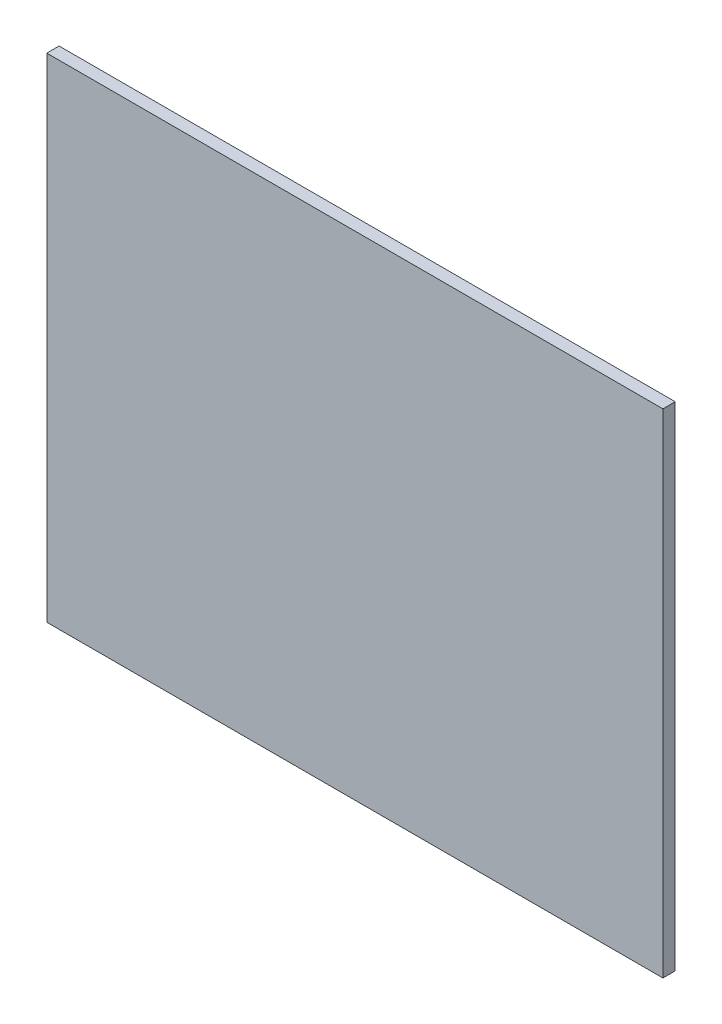
SolidWorks part; units mm, degrees
ref_plane "Front plane" through (0, 0, 0) normal (0, 0, 1) x (1, 0, 0)
ref_plane "Top plane" through (0, 0, 0) normal (0, 1, 0) x (1, 0, 0)
ref_plane "Right plane" through (0, 0, 0) normal (1, 0, 0) x (0, 0, -1)
sketch "Sketch1" plane through (0, 0, 0) normal (0, 0, 1) x (1, 0, 0)
  line L1 (-50, 40) -> (50, 40)
  line L2 (-50, 40) -> (-50, -40)
  line L3 (-50, -40) -> (50, -40)
  line L4 (50, 40) -> (50, -40)
  line L5 (-50, 40) -> (50, -40) construction
  line L6 (-50, -40) -> (50, 40) construction
  point P0 (0, 0)
  dimension "D1" = 100
  dimension "D2" = 80
extrude "Boss-Extrude1" add sketch "Sketch1" along normal blind 2
